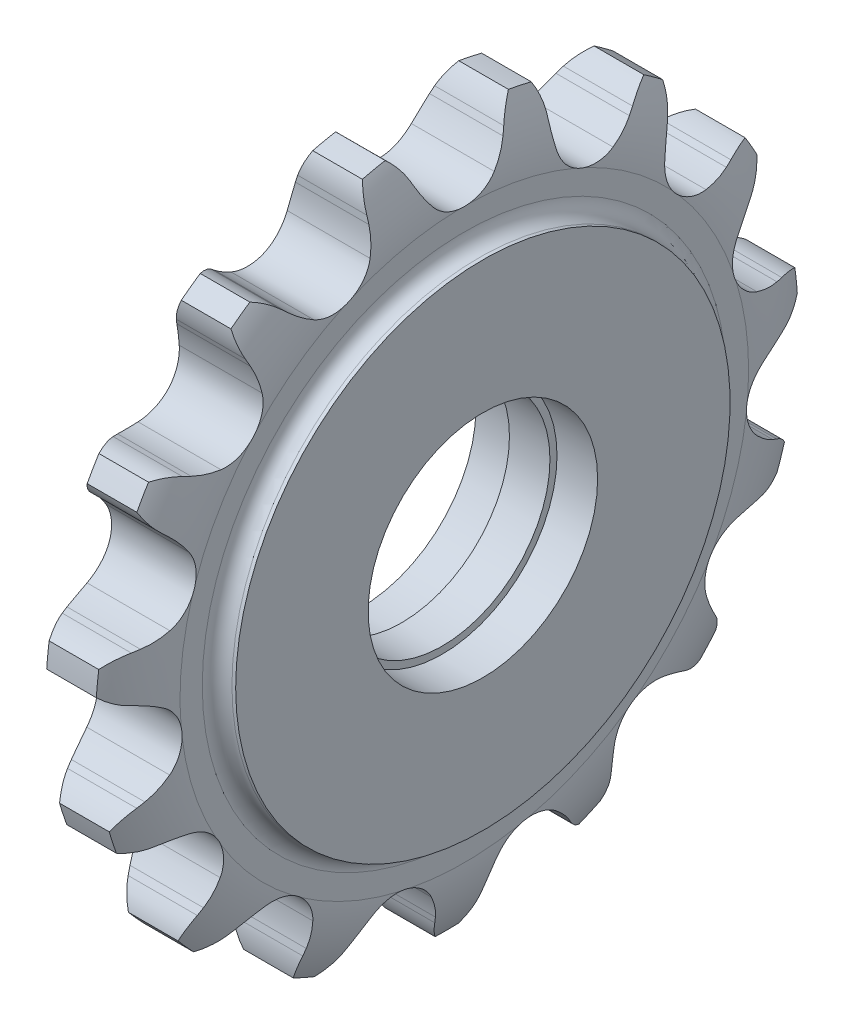
from build123d import *

# Parameters (mm, degrees)
EXTRUDECUTONE_DEPTH     = 16.984719634
PATTERNONE_COUNT        = 15
CUT_EXTRUDEA_DEPTH      = 142.587656458
CUT_EXTRUDEA_DEPTH_BACK = 142.587656458
SKETCHHOLE_R            = 15
CUT_EXTRUDEB_DEPTH      = 142.587656458
CUT_EXTRUDEB_DEPTH_BACK = 142.587656458
SKETCHKEY_W             = 8
SKETCHKEY_H             = 10.799999952
SKETCH_3_R              = 30.5
CUT_EXTRUDE_3_DEPTH     = 145.700280386
SKETCH_4_R              = 32.5
CUT_EXTRUDE_4_DEPTH     = 11.5


with BuildPart() as part:
    # Sketch1 → Revolve 2 (revolve)
    with BuildSketch(Plane.XY, mode=Mode.PRIVATE) as revolve_2_sk:
        with BuildLine():
            Line((-17.234719634, 0), (-17.234719634, 70))
            Line((-17.234719634, 70), (-16.183675707, 70))
            ThreePointArc((-16.183675707, 70), (-13.210874555, 71.231374555), (-11.9795, 74.204175707))
            Line((-11.9795, 74.204175707), (-11.9795, 80.510439267))
            ThreePointArc((-11.9795, 80.510439267), (-10.746639243, 90.329594971), (-7.0265, 99.5))
            Line((-7.0265, 99.5), (7.0265, 99.5))
            ThreePointArc((7.0265, 99.5), (10.746639243, 90.329594971), (11.9795, 80.510439267))
            Line((11.9795, 80.510439267), (11.9795, 74.204175707))
            ThreePointArc((11.9795, 74.204175707), (13.210874555, 71.231374555), (16.183675707, 70))
            Line((16.183675707, 70), (17.234719634, 70))
            Line((17.234719634, 70), (17.234719634, 0))
            Line((17.234719634, 0), (-17.234719634, 0))
        make_face()
    revolve(revolve_2_sk.sketch.rotate(Axis((-4, 0, 0), (1, 0, 0)), 90), axis=Axis((-4, 0, 0), (1, 0, 0)))

    # Sketch2 → ExtrudeCutOne (cut, symmetric)
    with BuildSketch(Plane(origin=(0, 0, 0), x_dir=(0, 0, -1), z_dir=(1, 0, 0))):
        with BuildLine():
            Line((12.523074172, 90.681887943), (13.354481298, 92.486730089))
            ThreePointArc((13.354481298, 92.486730089), (15.10924996, 95.437983979), (17.439423475, 97.959769849))
            ThreePointArc((17.439423475, 97.959769849), (0, 99.5), (-17.439423475, 97.959769849))
            ThreePointArc((-17.439423475, 97.959769849), (-15.10924996, 95.437983979), (-13.354481298, 92.486730089))
            Line((-13.354481298, 92.486730089), (-12.523074172, 90.681887943))
            ThreePointArc((-12.523074172, 90.681887943), (-10.812212003, 87.504472082), (-8.720024546, 84.564102621))
            ThreePointArc((-8.720024546, 84.564102621), (0, 80.404864267), (8.720024546, 84.564102621))
            ThreePointArc((8.720024546, 84.564102621), (10.812212003, 87.504472082), (12.523074172, 90.681887943))
        make_face()
    extrudecutone = extrude(amount=EXTRUDECUTONE_DEPTH, both=True, mode=Mode.SUBTRACT)

    # PatternOne: ExtrudeCutOne ×15 about axis
    patternone_axis = Axis((0, 0, 0), (1, 0, 0))
    for i in range(1, PATTERNONE_COUNT):
        add(extrudecutone.rotate(patternone_axis, i * 360 / PATTERNONE_COUNT), mode=Mode.SUBTRACT)

    # SketchHole → Cut-ExtrudeA (cut, two sides: drawn at the far end of the back side and taken through both)
    with BuildSketch(Plane(origin=(0, 0, 0), x_dir=(0, 0, -1), z_dir=(1, 0, 0)).offset(-CUT_EXTRUDEA_DEPTH_BACK)):
        Circle(SKETCHHOLE_R)
    extrude(amount=CUT_EXTRUDEA_DEPTH + CUT_EXTRUDEA_DEPTH_BACK, mode=Mode.SUBTRACT)

    # SketchKey → Cut-ExtrudeB (cut, two sides: drawn at the far end of the back side and taken through both)
    with BuildSketch(Plane(origin=(0, 0, 0), x_dir=(0, 0, -1), z_dir=(1, 0, 0)).offset(-CUT_EXTRUDEB_DEPTH_BACK)):
        with Locations((0, 12.899999976)):
            Rectangle(SKETCHKEY_W, SKETCHKEY_H)
    extrude(amount=CUT_EXTRUDEB_DEPTH + CUT_EXTRUDEB_DEPTH_BACK, mode=Mode.SUBTRACT)

    # 草图3 → 切除-拉伸3 (cut, through all)
    with BuildSketch(Plane(origin=(17.234719634, 0, 0), x_dir=(0, 0, -1), z_dir=(1, 0, 0))):
        Circle(SKETCH_3_R)
    extrude(amount=-CUT_EXTRUDE_3_DEPTH, mode=Mode.SUBTRACT)

    # 草图4 → 切除-拉伸4 (cut)
    with BuildSketch(Plane(origin=(17.234719634, 0, 0), x_dir=(0, 0, -1), z_dir=(1, 0, 0))):
        Circle(SKETCH_4_R)
    cut_extrude_4 = extrude(amount=-CUT_EXTRUDE_4_DEPTH, mode=Mode.SUBTRACT)

    # 镜向1: 切除-拉伸4 across plane
    add(cut_extrude_4.mirror(Plane(origin=(0, 0, 0), x_dir=(0, 0, 1), z_dir=(1, 0, 0))), mode=Mode.SUBTRACT)


solid = part.part
